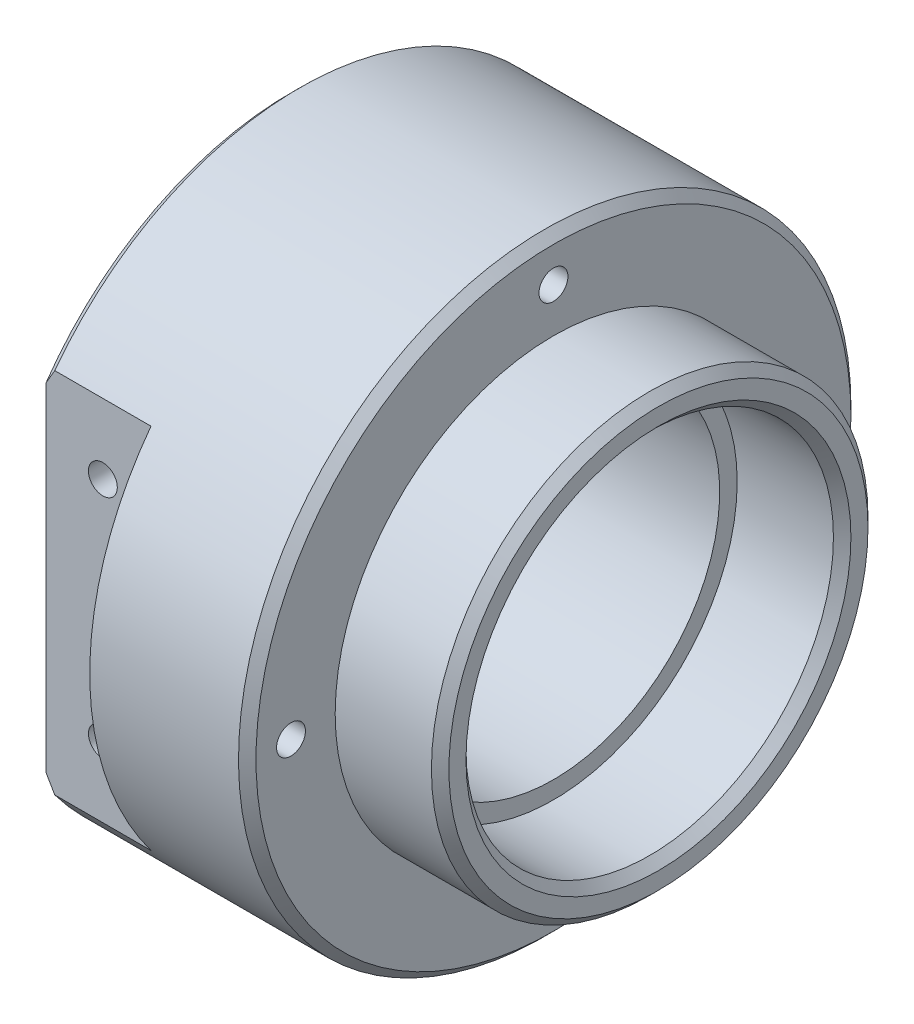
SolidWorks part; units mm, degrees
ref_plane "Front" through (0, 0, 0) normal (0, 0, 1) x (1, 0, 0)
ref_plane "Top" through (0, 0, 0) normal (0, 1, 0) x (1, 0, 0)
ref_plane "Right" through (0, 0, 0) normal (1, 0, 0) x (0, 0, -1)
sketch "Sketch1" plane through (0, 0, 0) normal (1, 0, 0) x (0, 0, -1)
  circle A0 centre (0, 0) radius 35
  dimension "D1" = 70
extrude "Boss-Extrude1" add sketch "Sketch1" along normal blind 20
sketch "Sketch2" plane through (20, 0, 0) normal (1, 0, 0) x (0, 0, -1)
  circle A0 centre (0, 0) radius 35
  dimension "D1" = 70
extrude "Boss-Extrude2" add sketch "Sketch2" along normal blind 10
sketch "Sketch3" plane through (30, 0, 0) normal (1, 0, 0) x (0, 0, -1)
  circle A0 centre (0, 0) radius 24.95
  dimension "D1" = 49.9
extrude "Boss-Extrude3" add sketch "Sketch3" along normal blind 12
sketch "Sketch4" plane through (0, 0, 0) normal (-1, 0, 0) x (0, 0, 1)
  circle A0 centre (0, 0) radius 21
  dimension "D1" = 42
extrude "Cut-Extrude1" cut sketch "Sketch4" against normal blind 12
sketch "Sketch5" plane through (12, 0, 0) normal (-1, 0, 0) x (0, 0, 1)
  circle A0 centre (0, 0) radius 19
  dimension "D1" = 38
extrude "Cut-Extrude2" cut sketch "Sketch5" against normal blind 18
sketch "Sketch6" plane through (30, 0, 0) normal (-1, 0, 0) x (0, 0, 1)
  circle A0 centre (0, 0) radius 21
  dimension "D1" = 42
extrude "Cut-Extrude3" cut sketch "Sketch6" against normal blind 28
hole_wizard "M4 Tapped Hole2" positions "Sketch8" profile "Sketch7" tap size "M4" standard "Gb"
sketch "Sketch8" plane through (30, 0, 0) normal (1, 0, 0) x (0, 0, -1)
  line L0 (0, 0) -> (35, 0) construction
  circle A0 centre (0, 0) radius 35 construction
  point P0 (30, 0)
  dimension "D1" = 30
sketch "Sketch7" plane through (30, 0, -30) normal (0, 1, 0) x (0, 0, -1)
  line L0 (0, 0) -> (0, 11.0914)
  line L1 (0, 11.0914) -> (1.65, 10.1)
  line L2 (1.65, 10.1) -> (1.65, 0)
  line L5 (1.65, 0) -> (0, 0)
  line L10 (0, 11.0914) -> (-1.65, 10.1) construction
  line L11 (0, -6.35) -> (0, 107.95) construction
  dimension "螺纹孔钻头直径" = 3.3
  dimension "螺纹孔钻头深度" = 10.1
  dimension "导头角度" = 118
cosmetic thread "Cosmetic Thread2" parameters "D1"=8, "D2"=4
pattern_circular "CirPattern1" count 4 every 90 about axis through (0, 0, 0) along (1, 0, 0) of "M4 Tapped Hole2"
sketch "Sketch9" plane through (0, 0, 0) normal (-1, 0, 0) x (0, 0, 1)
  line L1 (110.9258, -39.8142) -> (28, -39.8142)
  line L2 (110.9258, -39.8142) -> (110.9258, 39.8142)
  line L3 (110.9258, 39.8142) -> (28, 39.8142)
  line L4 (28, -39.8142) -> (28, 39.8142)
  line L5 (110.9258, -39.8142) -> (28, 39.8142) construction
  line L6 (110.9258, 39.8142) -> (28, -39.8142) construction
  point P0 (69.4629, 0)
  dimension "D1" = 28
extrude "Cut-Extrude4" cut sketch "Sketch9" against normal blind 12
hole_wizard "M4 Tapped Hole3" positions "Sketch11" profile "Sketch10" tap size "M4" standard "Gb"
sketch "Sketch11" plane through (0, 0, 28) normal (0, 0, 1) x (1, 0, 0)
  line L0 (0, 0) -> (49.996, 0) construction
  line L2 (0, -21) -> (0, 21) construction
  point P0 (6.5, 13)
  point P2 (6.5, -13)
  dimension "D1" = 26
  dimension "D2" = 6.5
sketch "Sketch10" plane through (6.5, 13, 28) normal (1, 0, 0) x (0, -1, 0)
  line L0 (0, 0) -> (0, 11.0914)
  line L1 (0, 11.0914) -> (1.65, 10.1)
  line L2 (1.65, 10.1) -> (1.65, 0)
  line L5 (1.65, 0) -> (0, 0)
  line L10 (0, 11.0914) -> (-1.65, 10.1) construction
  line L11 (0, -6.35) -> (0, 107.95) construction
  dimension "螺纹孔钻头直径" = 3.3
  dimension "螺纹孔钻头深度" = 10.1
  dimension "导头角度" = 118
cosmetic thread "Cosmetic Thread3" parameters "D1"=8, "D2"=4
cosmetic thread "Cosmetic Thread4" parameters "D1"=8, "D2"=4
chamfer "Chamfer1" distance 1 angle 45 5 edges at (0, 0, 21) (42, 0, -21) (42, 0, -24.95) (30, 0, -35) (0, 0, -35)
